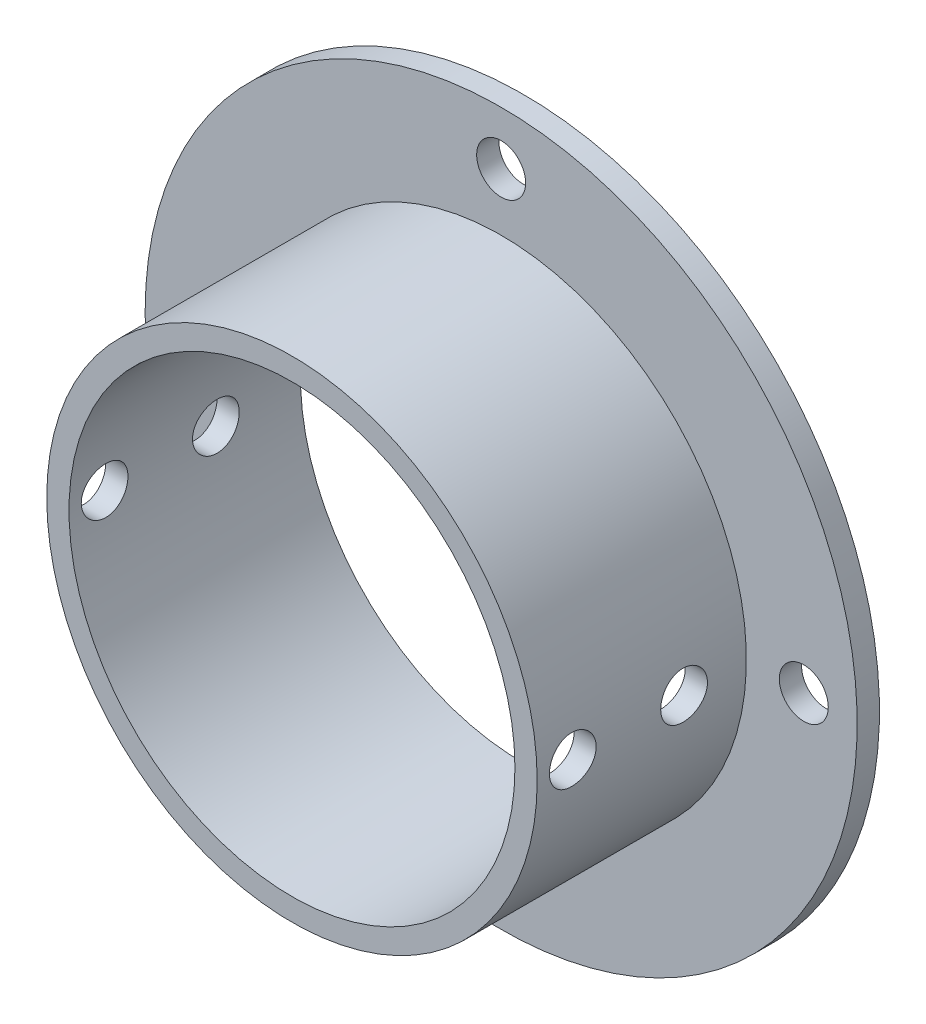
SolidWorks part; units mm, degrees
ref_plane "前视基准面" through (0, 0, 0) normal (0, 0, 1) x (1, 0, 0)
ref_plane "上视基准面" through (0, 0, 0) normal (0, 1, 0) x (1, 0, 0)
ref_plane "右视基准面" through (0, 0, 0) normal (1, 0, 0) x (0, 0, -1)
sketch "草图1" plane through (0, 0, 0) normal (0, 0, 1) x (1, 0, 0)
  circle A0 centre (0, 0) radius 55.1
  circle A1 centre (0, 0) radius 50.1
  dimension "D1" = 100.2
  dimension "D2" = 5
extrude "凸台-拉伸1" add sketch "草图1" along normal blind 52
sketch "草图2" plane through (0, 0, 0) normal (0, 0, -1) x (-1, 0, 0)
  circle A0 centre (0, 0) radius 80
  dimension "D1" = 160
extrude "凸台-拉伸2" add sketch "草图2" against normal blind 5
sketch "草图3" plane through (0, 0, 5) normal (0, 0, 1) x (1, 0, 0)
  line L0 (0, 80) -> (0, 56) construction
  circle A1 centre (0, 0) radius 80 construction
  circle A2 centre (0, 68) radius 5.5
  dimension "D1" = 11
  dimension "D2" = 68
extrude "切除-拉伸1" cut sketch "草图3" against normal blind 14
pattern_circular "阵列(圆周)1" count 4 over 360 about axis through (0, 0, 0) along (0, 0, 1) of "切除-拉伸1"
sketch "草图4" plane through (0, 0, 5) normal (0, 0, 1) x (1, 0, 0)
  circle A1 centre (0, 0) radius 50.1
  circle A6 centre (0, 0) radius 50.1
  dimension "D1" = 0
extrude "切除-拉伸2" cut sketch "草图4" against normal blind 66
sketch "草图6" plane through (0, 0, 0) normal (1, 0, 0) x (0, -1, 0)
  line L0 (0, -5) -> (0, -19) construction
  line L1 (-55.1, -5) -> (55.1, -5) construction
  line L2 (0, -19) -> (0, -44) construction
  circle A0 centre (0, -19) radius 5.25
  circle A1 centre (0, -44) radius 5.25
  dimension "D3" = 10.5
  dimension "D1" = 25
  dimension "D2" = 14
extrude "切除-拉伸3" cut sketch "草图6" against normal mid plane 206
